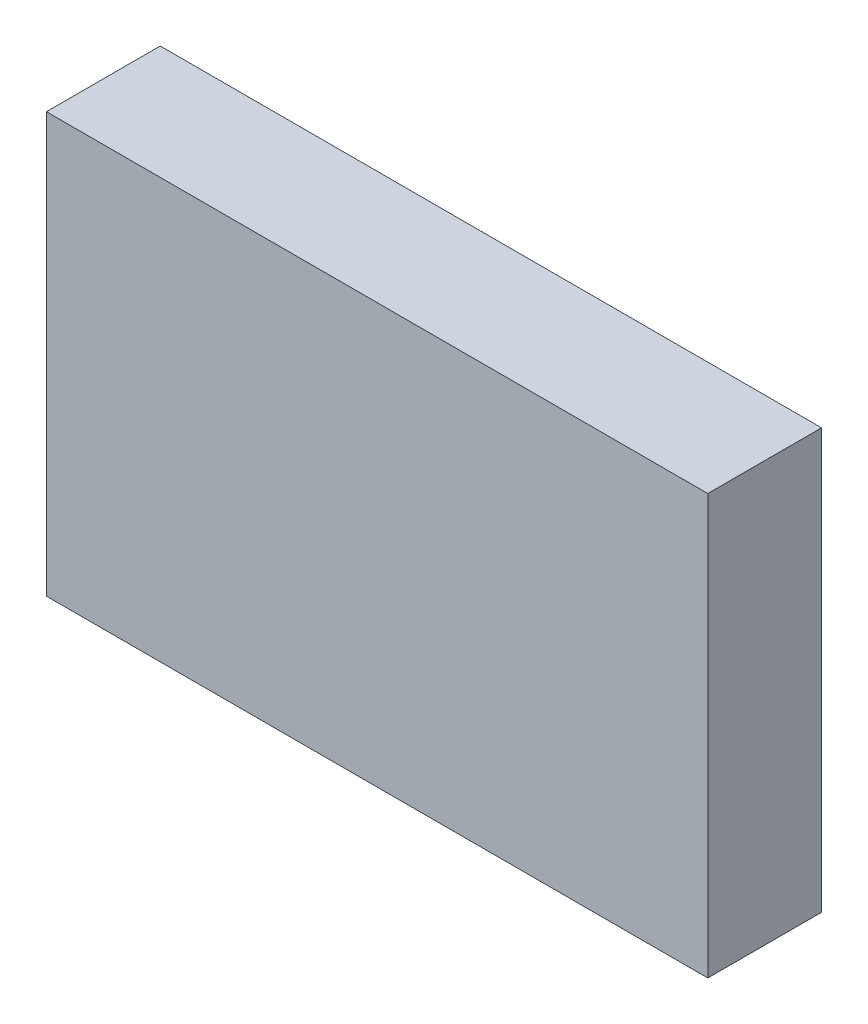
from build123d import *

# Parameters (mm, degrees)
SKETCH_1_W      = 465
SKETCH_1_H      = 295
EXTRUDE_1_DEPTH = 80


with BuildPart() as part:
    # 草图1 → 凸台-拉伸1 (new body)
    with BuildSketch(Plane.XY):
        Rectangle(SKETCH_1_W, SKETCH_1_H)
    extrude(amount=EXTRUDE_1_DEPTH)


solid = part.part
